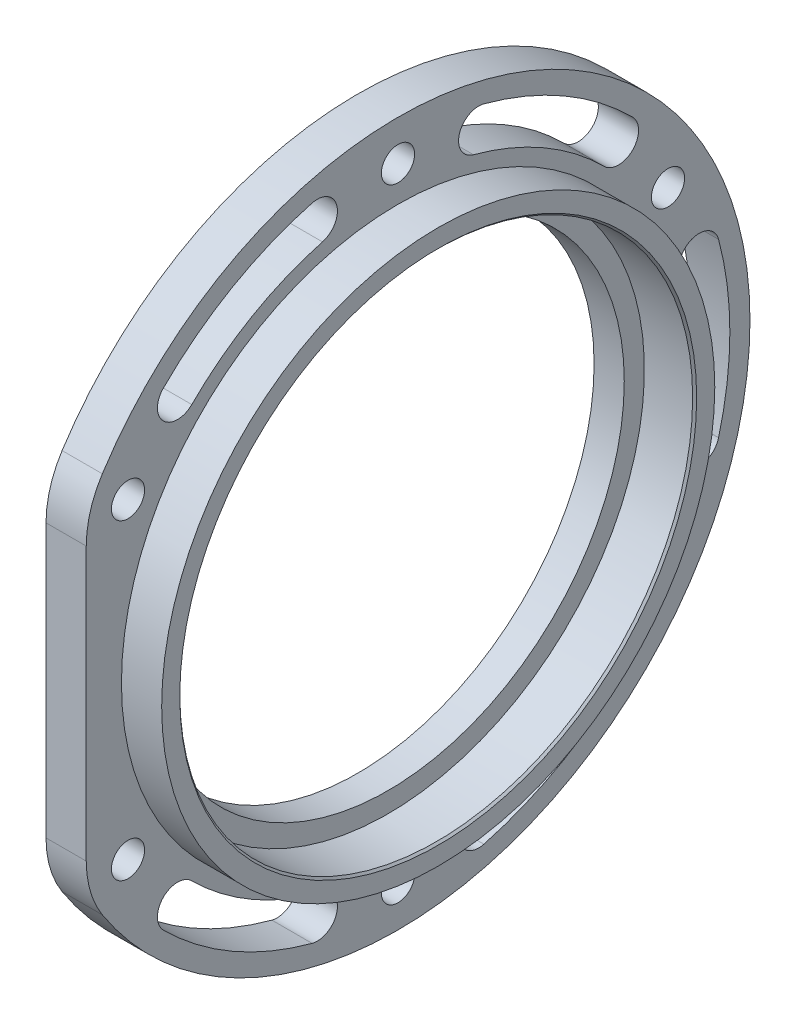
from build123d import *

# Parameters (mm, degrees)
HOLE_WIZARD_M4_1_D  = 3.3
CUT_EXTRUDE_1_DEPTH = 10
FILLET_1_R          = 10
CUT_EXTRUDE_2_DEPTH = 10
CHAMFER_1_SIZE      = 0.2


with BuildPart() as part:
    # 草图1 → 旋转1 (revolve)
    with BuildSketch(Plane(origin=(0, 0, 0), x_dir=(1, 0, 0), z_dir=(0, 1, 0)), mode=Mode.PRIVATE) as revolve_1_sk:
        Polygon((0, 23.5), (0, 35), (4, 35), (4, 27.5), (8, 27.5), (8, 25.5), (3, 25.5), (3, 23.5), align=None)
    revolve(revolve_1_sk.sketch.rotate(Axis((-554.392054902, 0, 0), (1, 0, 0)), 180), axis=Axis((-554.392054902, 0, 0), (1, 0, 0)))

    # M4 螺纹孔1 (through all)
    with Locations(Plane(origin=(4, 0, 0), x_dir=(0, 0, -1), z_dir=(1, 0, 0))):
        with Locations((0, 0), (0, 31), (26.846787517, 15.5), (26.846787517, -15.5), (0, -31), (-26.846787517, -15.5), (-26.846787517, 15.5)):
            Hole(HOLE_WIZARD_M4_1_D / 2)

    # 草图4 → 切除-拉伸1 (cut)
    with BuildSketch(Plane(origin=(4, 0, 0), x_dir=(0, 0, -1), z_dir=(1, 0, 0))):
        with BuildLine():
            Line((-31, -16.248076809), (-31, 16.248076809))
            ThreePointArc((-31, 16.248076809), (-35, 0), (-31, -16.248076809))
        make_face()
    extrude(amount=-CUT_EXTRUDE_1_DEPTH, mode=Mode.SUBTRACT)

    # 圆角1
    fillet_1_edges = [part.edges().sort_by_distance(p)[0] for p in [
        (2, 16.248076809, 31),
        (2, -16.248076809, 31),
    ]]
    fillet(fillet_1_edges, radius=FILLET_1_R)

    # 草图5 → 切除-拉伸2 (cut)
    with BuildSketch(Plane(origin=(4, 0, 0), x_dir=(0, 0, -1), z_dir=(1, 0, 0))):
        with BuildLine():
            ThreePointArc((23.334523779, 23.334523779), (16.5, 28.578838325), (8.541028488, 31.875552268))
            ThreePointArc((8.541028488, 31.875552268), (6.091538746, 30.461338705), (7.505752308, 28.011848962))
            ThreePointArc((7.505752308, 28.011848962), (14.5, 25.11473671), (20.506096654, 20.506096654))
            ThreePointArc((20.506096654, 20.506096654), (23.334523779, 20.506096654), (23.334523779, 23.334523779))
        make_face()
        with BuildLine():
            ThreePointArc((31.875552268, -8.541028488), (33, 0), (31.875552268, 8.541028488))
            ThreePointArc((31.875552268, 8.541028488), (29.426062525, 9.955242051), (28.011848962, 7.505752308))
            ThreePointArc((28.011848962, 7.505752308), (29, 0), (28.011848962, -7.505752308))
            ThreePointArc((28.011848962, -7.505752308), (29.426062525, -9.955242051), (31.875552268, -8.541028488))
        make_face()
        with BuildLine():
            ThreePointArc((8.541028488, -31.875552268), (16.5, -28.578838325), (23.334523779, -23.334523779))
            ThreePointArc((23.334523779, -23.334523779), (23.334523779, -20.506096654), (20.506096654, -20.506096654))
            ThreePointArc((20.506096654, -20.506096654), (14.5, -25.11473671), (7.505752308, -28.011848962))
            ThreePointArc((7.505752308, -28.011848962), (6.091538746, -30.461338705), (8.541028488, -31.875552268))
        make_face()
        with BuildLine():
            ThreePointArc((-23.334523779, -23.334523779), (-16.5, -28.578838325), (-8.541028488, -31.875552268))
            ThreePointArc((-8.541028488, -31.875552268), (-6.091538746, -30.461338705), (-7.505752308, -28.011848962))
            ThreePointArc((-7.505752308, -28.011848962), (-14.5, -25.11473671), (-20.506096654, -20.506096654))
            ThreePointArc((-20.506096654, -20.506096654), (-23.334523779, -20.506096654), (-23.334523779, -23.334523779))
        make_face()
        with BuildLine():
            ThreePointArc((-8.541028488, 31.875552268), (-16.5, 28.578838325), (-23.334523779, 23.334523779))
            ThreePointArc((-23.334523779, 23.334523779), (-23.334523779, 20.506096654), (-20.506096654, 20.506096654))
            ThreePointArc((-20.506096654, 20.506096654), (-14.5, 25.11473671), (-7.505752308, 28.011848962))
            ThreePointArc((-7.505752308, 28.011848962), (-6.091538746, 30.461338705), (-8.541028488, 31.875552268))
        make_face()
    extrude(amount=-CUT_EXTRUDE_2_DEPTH, mode=Mode.SUBTRACT)

    # 倒角1
    chamfer_1_edges = [part.edges().sort_by_distance(p)[0] for p in [
        (8, 0, -25.5),
    ]]
    chamfer(chamfer_1_edges, length=CHAMFER_1_SIZE)


solid = part.part
